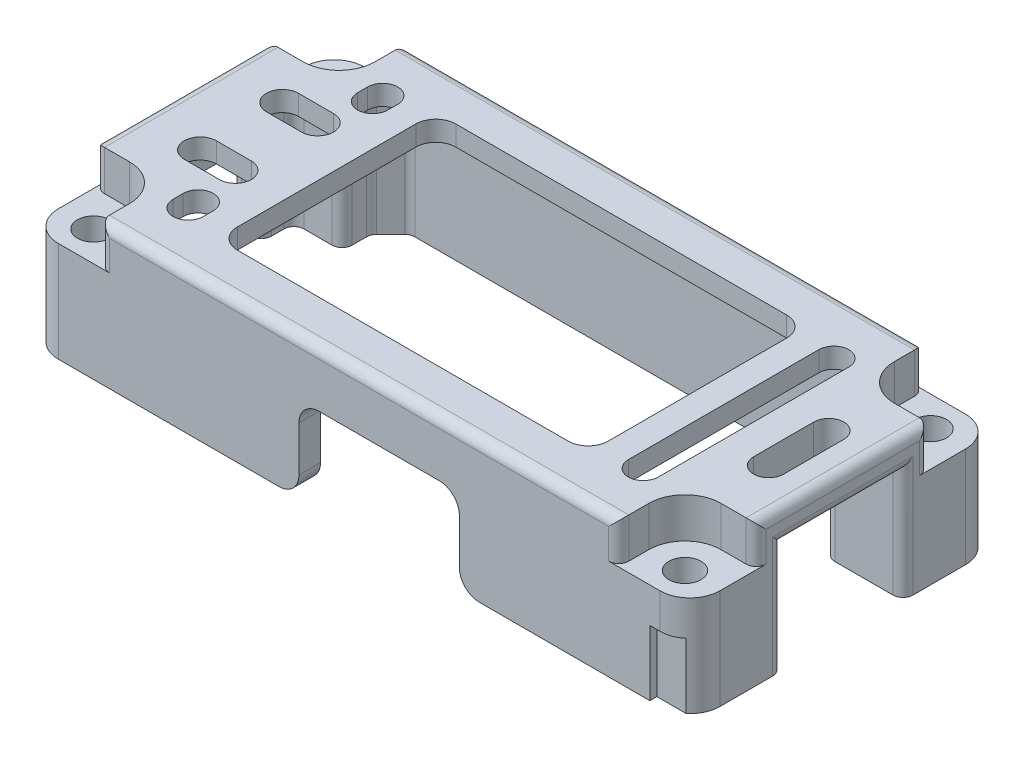
from build123d import *

# Parameters (mm, degrees)
SKETCH1_R              = 1.6
BOSS_EXTRUDE1_DEPTH    = 12
SKETCH2_W              = 52
SKETCH2_H              = 26.2
CUT_EXTRUDE1_DEPTH     = 2
SKETCH3_W              = 7.4
SKETCH3_H              = 20
CUT_EXTRUDE2_DEPTH     = 8
SKETCH4_W              = 16
SKETCH4_H              = 4.5
CUT_EXTRUDE3_DEPTH     = 2.15
SKETCH5_W              = 52
SKETCH5_H              = 26.2
CUT_EXTRUDE4_DEPTH     = 39.28266579
SKETCH6_W              = 66
SKETCH6_H              = 30.5
SKETCH6_R              = 1.6
SKETCH6_W_2            = 37
SKETCH6_H_2            = 21.8
BOSS_EXTRUDE2_DEPTH    = 2
SKETCH7_W              = 2
SKETCH7_H              = 12
SKETCH7_W_2            = 1.6
SKETCH7_H_2            = 8
CUT_EXTRUDE5_DEPTH     = 39.28266579
SKETCH8_W              = 16
SKETCH8_H              = 2.15
CUT_EXTRUDE6_DEPTH     = 38.33379836
SKETCH9_W              = 0.8
SKETCH9_H              = 7.1
BOSS_EXTRUDE3_DEPTH    = 12
CUT_EXTRUDE7_DEPTH     = 12
SKETCH11_W             = 3
SKETCH11_H             = 10
BOSS_EXTRUDE4_DEPTH    = 3
SKETCH13_W             = 7.8
SKETCH13_H             = 12
BOSS_EXTRUDE5_DEPTH    = 1
CHAMFER1_SIZE          = 2
CUT_EXTRUDE8_DEPTH     = 4
CUT_EXTRUDE9_DEPTH     = 39.955904559
R1_TRANSITION_FILLET_R = 1
R2_TRANSITION_FILLET_R = 2
R3_TRANSITION_FILLET_R = 3
CUT_EXTRUDE10_START    = -6.5
CUT_EXTRUDE10_DEPTH    = 6.5


with BuildPart() as part:
    # Sketch1 → Boss-Extrude1 (new body)
    with BuildSketch(Plane(origin=(0, 0, 0), x_dir=(1, 0, 0), z_dir=(0, 1, 0))):
        Polygon((-33, 4), (-27.6, 4), (-27.6, -4), (-33, -4), (-33, -15.25), (33, -15.25), (33, -6), (28, -6), (28, 6), (33, 6), (33, 15.25), (-33, 15.25), align=None)
        with Locations(Location((-29.5, 12.25, 0), (0, 0, 270))):
            Circle(SKETCH1_R, mode=Mode.SUBTRACT)
        with Locations(Location((29.5, 12.25, 0), (0, 0, 270))):
            Circle(SKETCH1_R, mode=Mode.SUBTRACT)
        with Locations(Location((-29.5, -12.25, 0), (0, 0, 90))):
            Circle(SKETCH1_R, mode=Mode.SUBTRACT)
        with Locations(Location((29.5, -12.25, 0), (0, 0, 90))):
            Circle(SKETCH1_R, mode=Mode.SUBTRACT)
        Polygon((-26, -5.75), (-26, 5.75), (-21.1, 5.75), (-21.1, 13.1), (21.1, 13.1), (21.1, -13.1), (-21.1, -13.1), (-21.1, -5.75), align=None, mode=Mode.SUBTRACT)
    extrude(amount=BOSS_EXTRUDE1_DEPTH)

    # Sketch2 → Cut-Extrude1 (cut)
    with BuildSketch(Plane.XZ):
        Rectangle(SKETCH2_W, SKETCH2_H)
    extrude(amount=-CUT_EXTRUDE1_DEPTH, mode=Mode.SUBTRACT)

    # Sketch3 → Cut-Extrude2 (cut)
    with BuildSketch(Plane(origin=(0, 12, 0), x_dir=(1, 0, 0), z_dir=(0, 1, 0))):
        with Locations((-26.8, 0)):
            Rectangle(SKETCH3_W, SKETCH3_H)
        Polygon((28, -6), (28, 6), (26, 6), (26, 13.1), (21.1, 13.1), (21.1, -13.1), (26, -13.1), (26, -6), align=None)
    extrude(amount=-CUT_EXTRUDE2_DEPTH, mode=Mode.SUBTRACT)

    # Sketch4 → Cut-Extrude3 (cut)
    with BuildSketch(Plane.XY.offset(15.25)):
        with Locations((2, 6.25)):
            Rectangle(SKETCH4_W, SKETCH4_H)
    extrude(amount=-CUT_EXTRUDE3_DEPTH, mode=Mode.SUBTRACT)

    # Sketch5 → Cut-Extrude4 (cut, through all)
    with BuildSketch(Plane.XZ):
        Rectangle(SKETCH5_W, SKETCH5_H)
    extrude(amount=-CUT_EXTRUDE4_DEPTH, mode=Mode.SUBTRACT)

    # Sketch6 → Boss-Extrude2 (add)
    with BuildSketch(Plane(origin=(0, 12, 0), x_dir=(1, 0, 0), z_dir=(0, 1, 0))):
        Rectangle(SKETCH6_W, SKETCH6_H)
        with Locations(Location((-29.5, -12.25, 0), (0, 0, 90))):
            Circle(SKETCH6_R, mode=Mode.SUBTRACT)
        with Locations(Location((29.5, -12.25, 0), (0, 0, 90))):
            Circle(SKETCH6_R, mode=Mode.SUBTRACT)
        with Locations(Location((29.5, 12.25, 0), (0, 0, 270))):
            Circle(SKETCH6_R, mode=Mode.SUBTRACT)
        with Locations(Location((-29.5, 12.25, 0), (0, 0, 270))):
            Circle(SKETCH6_R, mode=Mode.SUBTRACT)
        Rectangle(SKETCH6_W_2, SKETCH6_H_2, mode=Mode.SUBTRACT)
    extrude(amount=BOSS_EXTRUDE2_DEPTH)

    # Sketch7 → Cut-Extrude5 (cut, through all)
    with BuildSketch(Plane.XZ.offset(-12)):
        with Locations((27, 0)):
            Rectangle(SKETCH7_W, SKETCH7_H)
        with Locations((-26.8, 0)):
            Rectangle(SKETCH7_W_2, SKETCH7_H_2)
    extrude(amount=CUT_EXTRUDE5_DEPTH, mode=Mode.SUBTRACT)

    # Sketch8 → Cut-Extrude6 (cut, through all)
    with BuildSketch(Plane.XZ.offset(-8.5)):
        with Locations((2, 14.175)):
            Rectangle(SKETCH8_W, SKETCH8_H)
    extrude(amount=CUT_EXTRUDE6_DEPTH, mode=Mode.SUBTRACT)

    # Sketch9 → Boss-Extrude3 (add, through all)
    with BuildSketch(Plane.XZ.offset(-12)):
        with Locations((25.6, 9.55)):
            Rectangle(SKETCH9_W, SKETCH9_H)
        Polygon((-25.2, -13.1), (-26, -13.1), (-26, -10), (-30.5, -10), (-30.5, -4), (-33, -4), (-33, 4), (-30.5, 4), (-30.5, 10), (-26, 10), (-26, 13.1), (-25.2, 13.1), align=None)
        with Locations((25.6, -9.55)):
            Rectangle(SKETCH9_W, SKETCH9_H)
    extrude(amount=BOSS_EXTRUDE3_DEPTH)

    # Sketch10 → Cut-Extrude7 (cut)
    with BuildSketch(Plane.XZ):
        Polygon((-33, -5), (-33, 5), (-30, 5), (-30, 8.25), (-25.2, 8.25), (-25.2, -8.25), (-30, -8.25), (-30, -5), align=None)
    extrude(amount=-CUT_EXTRUDE7_DEPTH, mode=Mode.SUBTRACT)

    # Sketch11 → Boss-Extrude4 (add)
    with BuildSketch(Plane.XZ.offset(-12)):
        with Locations((-31.5, 0)):
            Rectangle(SKETCH11_W, SKETCH11_H)
    extrude(amount=BOSS_EXTRUDE4_DEPTH)

    # Sketch13 → Boss-Extrude5 (add)
    with BuildSketch(Plane.XZ.offset(-12)):
        with Locations((29.1, 0)):
            Rectangle(SKETCH13_W, SKETCH13_H)
    extrude(amount=BOSS_EXTRUDE5_DEPTH)

    # Chamfer1
    chamfer1_edges = [part.edges().sort_by_distance(p)[0] for p in [
        (-25.2, 6, -13.1),
        (-25.2, 6, 13.1),
        (25.2, 6, 13.1),
        (25.2, 6, -13.1),
    ]]
    chamfer(chamfer1_edges, length=CHAMFER1_SIZE)

    # Sketch12 → Cut-Extrude8 (cut)
    with BuildSketch(Plane(origin=(0, 14, 0), x_dir=(1, 0, 0), z_dir=(0, 1, 0))):
        with BuildLine():
            Line((-29.5, 8.65), (-33, 8.65))
            Line((-33, 8.65), (-33, 15.25))
            Line((-33, 15.25), (-25.9, 15.25))
            Line((-25.9, 15.25), (-25.9, 12.25))
            ThreePointArc((-25.9, 12.25), (-26.954415588, 9.704415588), (-29.5, 8.65))
        make_face()
        with BuildLine():
            Line((29.5, 8.65), (33, 8.65))
            Line((33, 8.65), (33, 15.25))
            Line((33, 15.25), (25.9, 15.25))
            Line((25.9, 15.25), (25.9, 12.25))
            ThreePointArc((25.9, 12.25), (26.954415588, 9.704415588), (29.5, 8.65))
        make_face()
        with BuildLine():
            Line((29.5, -8.65), (33, -8.65))
            Line((33, -8.65), (33, -15.25))
            Line((33, -15.25), (25.9, -15.25))
            Line((25.9, -15.25), (25.9, -12.25))
            ThreePointArc((25.9, -12.25), (26.954415588, -9.704415588), (29.5, -8.65))
        make_face()
        with BuildLine():
            Line((-25.9, -12.25), (-25.9, -15.25))
            Line((-25.9, -15.25), (-33, -15.25))
            Line((-33, -15.25), (-33, -8.65))
            Line((-33, -8.65), (-29.5, -8.65))
            ThreePointArc((-29.5, -8.65), (-26.954415588, -9.704415588), (-25.9, -12.25))
        make_face()
    extrude(amount=-CUT_EXTRUDE8_DEPTH, mode=Mode.SUBTRACT)

    # Sketch14 → Cut-Extrude9 (cut, through all)
    with BuildSketch(Plane(origin=(0, 14, 0), x_dir=(1, 0, 0), z_dir=(0, 1, 0))):
        with BuildLine():
            Line((21.1, -9.5), (21.1, 9.5))
            ThreePointArc((21.1, 9.5), (22.6, 11), (24.1, 9.5))
            Line((24.1, 9.5), (24.1, -9.5))
            ThreePointArc((24.1, -9.5), (22.6, -11), (21.1, -9.5))
        make_face()
        with BuildLine():
            Line((27.1, -3), (27.1, 3))
            ThreePointArc((27.1, 3), (28.6, 4.5), (30.1, 3))
            Line((30.1, 3), (30.1, -3))
            ThreePointArc((30.1, -3), (28.6, -4.5), (27.1, -3))
        make_face()
        with BuildLine():
            Line((-27, 5.7), (-23.5, 5.7))
            ThreePointArc((-23.5, 5.7), (-21.9, 4.1), (-23.5, 2.5))
            Line((-23.5, 2.5), (-27, 2.5))
            ThreePointArc((-27, 2.5), (-28.6, 4.1), (-27, 5.7))
        make_face()
        with BuildLine():
            Line((-27, -5.7), (-23.5, -5.7))
            ThreePointArc((-23.5, -5.7), (-21.9, -4.1), (-23.5, -2.5))
            Line((-23.5, -2.5), (-27, -2.5))
            ThreePointArc((-27, -2.5), (-28.6, -4.1), (-27, -5.7))
        make_face()
        with BuildLine():
            Line((-21.1, 9.7), (-21.1, 8.7))
            ThreePointArc((-21.1, 8.7), (-22.6, 7.2), (-24.1, 8.7))
            Line((-24.1, 8.7), (-24.1, 9.7))
            ThreePointArc((-24.1, 9.7), (-22.6, 11.2), (-21.1, 9.7))
        make_face()
        with BuildLine():
            Line((-21.1, -9.7), (-21.1, -8.7))
            ThreePointArc((-21.1, -8.7), (-22.6, -7.2), (-24.1, -8.7))
            Line((-24.1, -8.7), (-24.1, -9.7))
            ThreePointArc((-24.1, -9.7), (-22.6, -11.2), (-21.1, -9.7))
        make_face()
    extrude(amount=-CUT_EXTRUDE9_DEPTH, mode=Mode.SUBTRACT)

    # R1 transition fillet
    r1_transition_fillet_edges = [part.edges().sort_by_distance(p)[0] for p in [
        (25.2, 5.5, 6),
        (25.2, 5.5, -6),
        (-30, 6, -8.25),
        (-25.2, 6, -8.25),
        (-25.2, 6, 8.25),
        (-30, 6, 8.25),
        (-30, 4.5, 5),
        (-33, 4.5, 5),
        (-30, 4.5, -5),
        (-33, 4.5, -5),
        (-33, 9, 0),
        (33, 5.5, 6),
        (33, 5.5, -6),
        (33, 11, 0),
        (-25.2, 6, -11.1),
        (23.2, 6, -13.1),
        (-23.2, 6, -13.1),
        (25.2, 6, 11.1),
        (25.2, 6, -11.1),
        (-23.2, 6, 13.1),
        (23.2, 6, 13.1),
        (-25.2, 6, 11.1),
        (0, 14, -15.25),
        (-33, 14, 0),
        (0, 14, 15.25),
        (33, 14, 0),
        (33, 12, 8.65),
        (25.9, 12, 15.25),
        (-25.9, 12, 15.25),
        (-33, 12, 8.65),
        (-33, 12, -8.65),
        (-25.9, 12, -15.25),
        (25.9, 12, -15.25),
        (33, 12, -8.65),
    ]]
    fillet(r1_transition_fillet_edges, radius=R1_TRANSITION_FILLET_R)

    # R2 transition fillet
    r2_transition_fillet_edges = [part.edges().sort_by_distance(p)[0] for p in [
        (10, 8.5, 14.175),
        (-6, 8.5, 14.175),
        (-18.5, 13, 10.9),
        (18.5, 13, 10.9),
        (18.5, 13, -10.9),
        (-18.5, 13, -10.9),
        (10, 0, 14.175),
        (-6, 0, 14.175),
    ]]
    fillet(r2_transition_fillet_edges, radius=R2_TRANSITION_FILLET_R)

    # R3 transition fillet
    r3_transition_fillet_edges = [part.edges().sort_by_distance(p)[0] for p in [
        (-33, 5, 15.25),
        (-33, 5, -15.25),
        (33, 5, -15.25),
        (33, 5, 15.25),
    ]]
    fillet(r3_transition_fillet_edges, radius=R3_TRANSITION_FILLET_R)

    # Sketch15 → Cut-Extrude10 (cut)
    with BuildSketch(Plane.XZ.offset(CUT_EXTRUDE10_START)):
        with BuildLine():
            Line((29, 15.25), (30, 15.25))
            ThreePointArc((30, 15.25), (31.024695077, 15.069574436), (31.926136028, 14.55))
            Line((31.926136028, 14.55), (29, 14.55))
            Line((29, 14.55), (29, 15.25))
        make_face()
    extrude(amount=CUT_EXTRUDE10_DEPTH, mode=Mode.SUBTRACT)


solid = part.part
